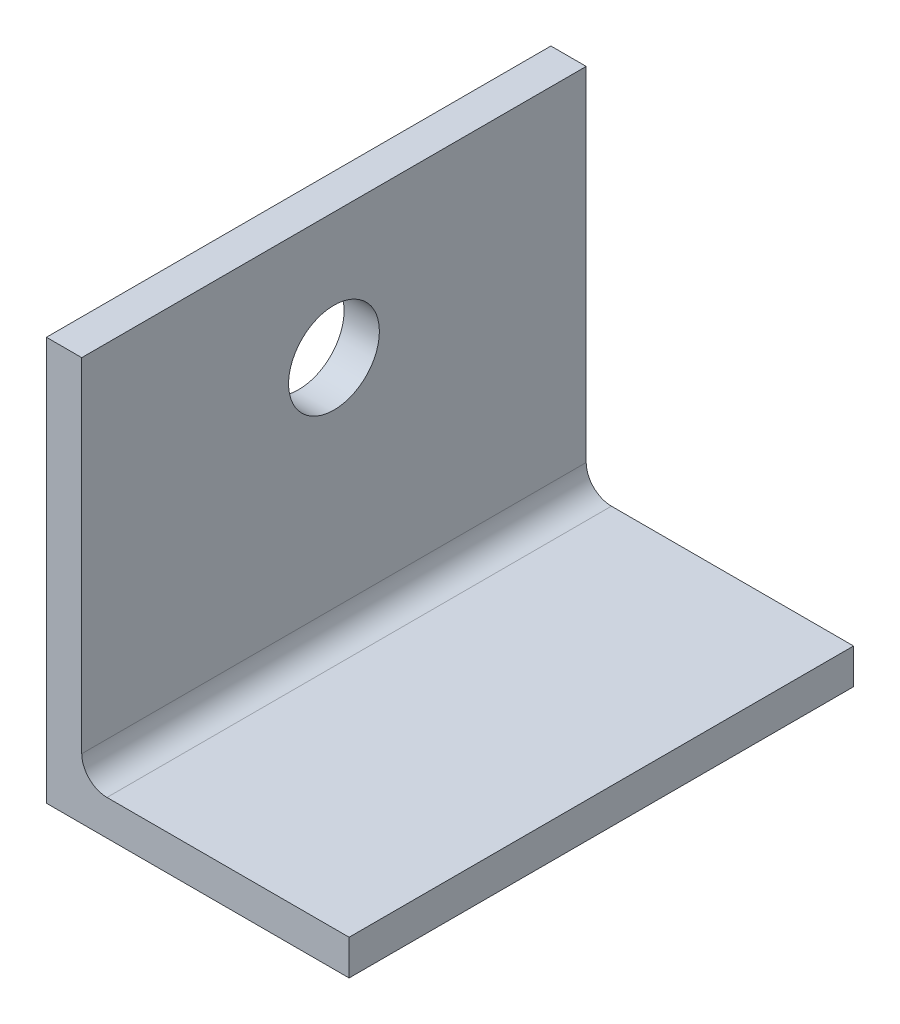
from build123d import *

# Parameters (mm, degrees)
BOSS_EXTRUDE1_DEPTH = 100
SKETCH2_R           = 9
CUT_EXTRUDE1_DEPTH  = 100
FILLET1_R           = 5


with BuildPart() as part:
    # Sketch1 → Boss-Extrude1 (new body)
    with BuildSketch(Plane.XY):
        Polygon((0, 0), (0, -80), (60, -80), (60, -73), (7, -73), (7, 0), align=None)
    extrude(amount=BOSS_EXTRUDE1_DEPTH)

    # Sketch2 → Cut-Extrude1 (cut)
    with BuildSketch(Plane(origin=(7, 0, 0), x_dir=(0, 0, -1), z_dir=(1, 0, 0))):
        with Locations((-50, -25)):
            Circle(SKETCH2_R)
    extrude(amount=-CUT_EXTRUDE1_DEPTH, mode=Mode.SUBTRACT)

    # Fillet1
    fillet1_edges = [part.edges().sort_by_distance(p)[0] for p in [
        (7, -73, 50),
    ]]
    fillet(fillet1_edges, radius=FILLET1_R)


solid = part.part
